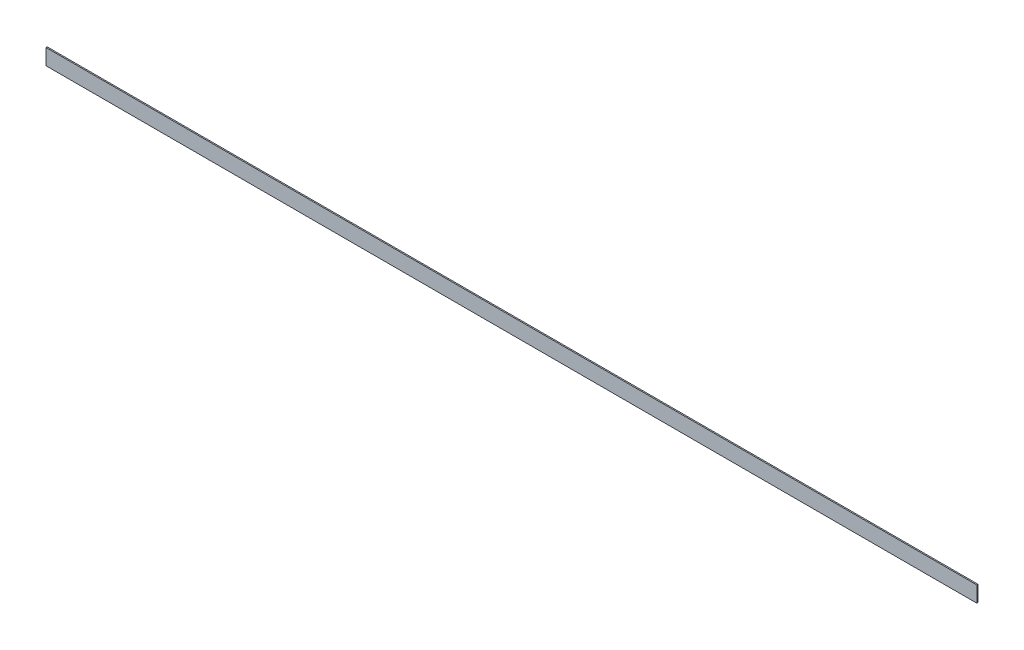
from build123d import *

# Parameters (mm, degrees)
SKETCH1_W           = 2350
SKETCH1_H           = 40
BOSS_EXTRUDE1_DEPTH = 3


with BuildPart() as part:
    # Sketch1 → Boss-Extrude1 (new body)
    with BuildSketch(Plane.XY):
        with Locations((1175, -20)):
            Rectangle(SKETCH1_W, SKETCH1_H)
    extrude(amount=BOSS_EXTRUDE1_DEPTH)


solid = part.part
